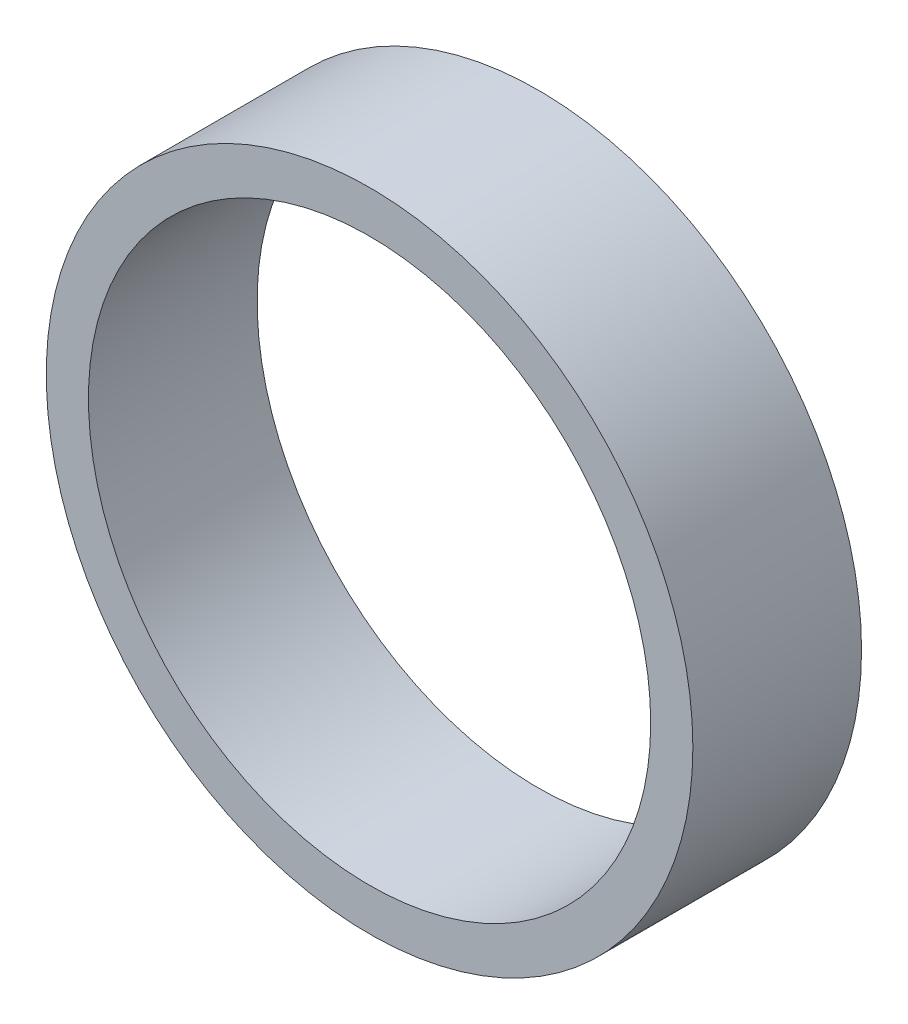
SolidWorks part; units mm, degrees
ref_plane "前视基准面" through (0, 0, 0) normal (0, 0, 1) x (1, 0, 0)
ref_plane "上视基准面" through (0, 0, 0) normal (0, 1, 0) x (1, 0, 0)
ref_plane "右视基准面" through (0, 0, 0) normal (1, 0, 0) x (0, 0, -1)
sketch "草图1" plane through (0, 0, 0) normal (0, 0, 1) x (1, 0, 0)
  circle A0 centre (0, 0) radius 20
  circle A1 centre (0, 0) radius 23
extrude "凸台-拉伸1" add sketch "草图1" along normal blind 12
